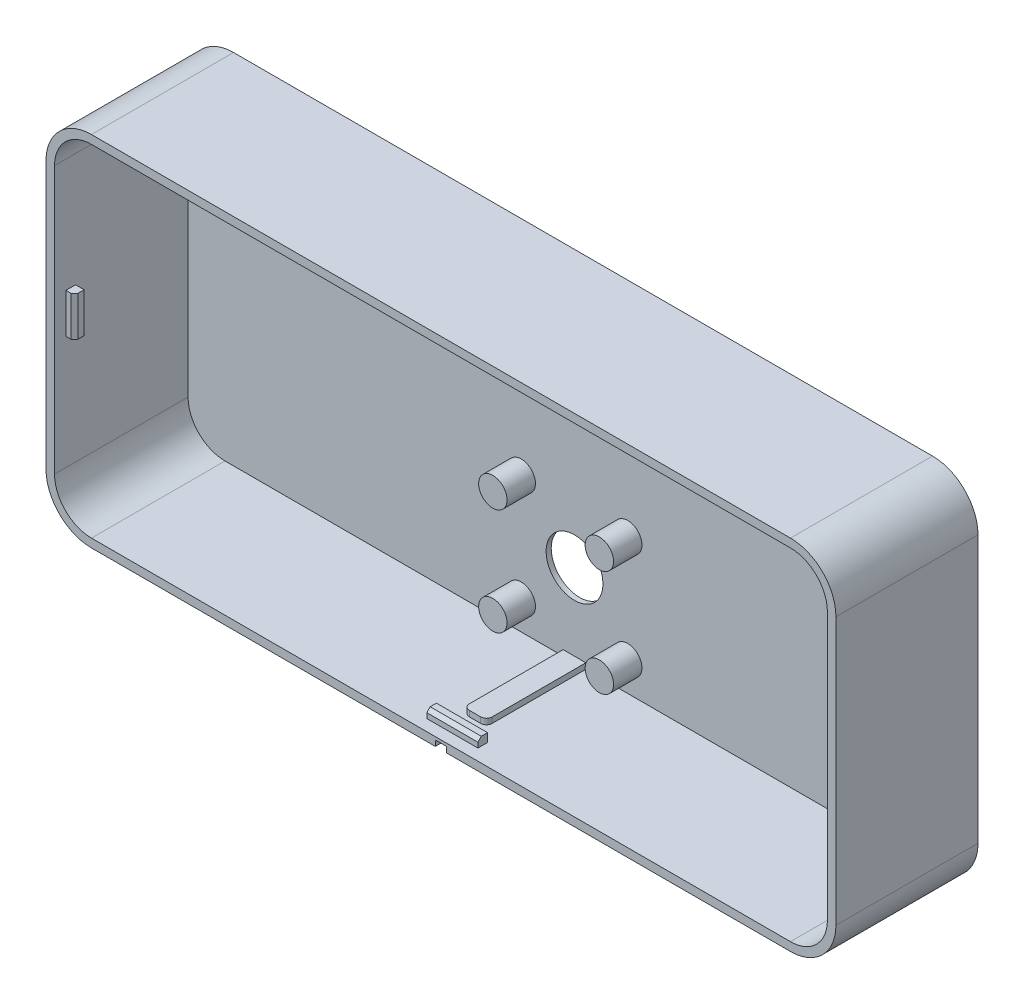
from build123d import *

# Parameters (mm, degrees)
BOSS_EXTRUDE1_DEPTH      = 25
SHELL1_T                 = -1.5
SKETCH2_W                = 9
SKETCH2_H                = 1.7
BOSS_EXTRUDE2_DEPTH      = 1.5
CHAMFER1_SIZE            = 0.6
CHAMFER1_OF_MIRROR1_SIZE = 0.6
SKETCH3_W                = 4
SKETCH3_H                = 17.5
BOSS_EXTRUDE3_DEPTH      = 1
SKETCH6_R                = 10.15
CUT_EXTRUDE3_DEPTH       = 0.6
SKETCH10_R               = 5
CUT_EXTRUDE4_DEPTH       = 81.111547233
SKETCH11_R               = 8
SKETCH11_R_2             = 7
BOSS_EXTRUDE5_DEPTH      = 0.6
SKETCH13_R               = 2.5
BOSS_EXTRUDE6_DEPTH      = 5
CUT_EXTRUDE5_START       = -2
SKETCH15_R               = 0.5
CUT_EXTRUDE5_DEPTH       = 77.515921952
SKETCH16_W               = 2
SKETCH16_H               = 58.164373892
CUT_EXTRUDE6_DEPTH       = 1
FILLET2_R                = 0.1
SKETCH17_R               = 15.5
SKETCH17_R_2             = 10.15
SKETCH17_R_3             = 0.5
BOSS_EXTRUDE7_DEPTH      = 1.2
SKETCH18_W               = 2
SKETCH18_H               = 1.626209188
CUT_EXTRUDE7_DEPTH       = 1
FILLET3_R                = 0.5
FILLET4_R                = 1
SKETCH19_W               = 1.7
SKETCH19_H               = 7
BOSS_EXTRUDE8_DEPTH      = 1.5
CHAMFER2_SIZE            = 0.6
CHAMFER2_OF_MIRROR2_SIZE = 0.6
FILLET5_R                = 0.2


with BuildPart() as part:
    # Sketch1 → Boss-Extrude1 (new body)
    with BuildSketch(Plane.XY):
        with BuildLine():
            Line((-61.5, 31.5), (61.5, 31.5))
            ThreePointArc((61.5, 31.5), (67.156854249, 29.156854249), (69.5, 23.5))
            Line((69.5, 23.5), (69.5, -23.5))
            ThreePointArc((69.5, -23.5), (67.156854249, -29.156854249), (61.5, -31.5))
            Line((61.5, -31.5), (-61.5, -31.5))
            ThreePointArc((-61.5, -31.5), (-67.156854249, -29.156854249), (-69.5, -23.5))
            Line((-69.5, -23.5), (-69.5, 23.5))
            ThreePointArc((-69.5, 23.5), (-67.156854249, 29.156854249), (-61.5, 31.5))
        make_face()
    extrude(amount=BOSS_EXTRUDE1_DEPTH)

    # Shell1
    shell1_openings = [part.faces().sort_by_distance(p)[0] for p in [
        (0, 0, 25),
    ]]
    offset(amount=SHELL1_T, openings=shell1_openings, kind=Kind.INTERSECTION)

    # Sketch2 → Boss-Extrude2 (add)
    with BuildSketch(Plane(origin=(0, 30, 0), x_dir=(-1, 0, 0), z_dir=(0, -1, 0))):
        with Locations((0, -22.15)):
            Rectangle(SKETCH2_W, SKETCH2_H)
    boss_extrude2 = extrude(amount=BOSS_EXTRUDE2_DEPTH)

    # Chamfer1
    chamfer1_edges = [part.edges().sort_by_distance(p)[0] for p in [
        (0, 28.5, 23),
    ]]
    chamfer(chamfer1_edges, length=CHAMFER1_SIZE)

    # Mirror1: Boss-Extrude2 across plane
    add(boss_extrude2.mirror(Plane.ZX))

    # Chamfer1 of Mirror1
    chamfer1_of_mirror1_edges = [part.edges().sort_by_distance(p)[0] for p in [
        (0, -28.5, 23),
    ]]
    chamfer(chamfer1_of_mirror1_edges, length=CHAMFER1_OF_MIRROR1_SIZE)

    # Sketch3 → Boss-Extrude3 (add)
    with BuildSketch(Plane(origin=(0, -30, 0), x_dir=(1, 0, 0), z_dir=(0, 1, 0))):
        with Locations((0, -10.25)):
            Rectangle(SKETCH3_W, SKETCH3_H)
    extrude(amount=BOSS_EXTRUDE3_DEPTH)

    # Sketch6 → Cut-Extrude3 (cut)
    with BuildSketch(Plane(origin=(0, 0, 0), x_dir=(-1, 0, 0), z_dir=(0, 0, -1))):
        with Locations((0, -15.5)):
            Circle(SKETCH6_R)
    extrude(amount=-CUT_EXTRUDE3_DEPTH, mode=Mode.SUBTRACT)

    # Sketch10 → Cut-Extrude4 (cut, through all)
    with BuildSketch(Plane(origin=(0, 0, 0.6), x_dir=(-1, 0, 0), z_dir=(0, 0, -1))):
        with Locations((0, -15.5)):
            Circle(SKETCH10_R)
    extrude(amount=-CUT_EXTRUDE4_DEPTH, mode=Mode.SUBTRACT)

    # Sketch11 → Boss-Extrude5 (add)
    with BuildSketch(Plane(origin=(0, 0, 0.6), x_dir=(-1, 0, 0), z_dir=(0, 0, -1))):
        with Locations((0, -15.5)):
            Circle(SKETCH11_R)
        with Locations((0, -15.5)):
            Circle(SKETCH11_R_2, mode=Mode.SUBTRACT)
    extrude(amount=BOSS_EXTRUDE5_DEPTH)

    # Sketch13 → Boss-Extrude6 (add)
    with BuildSketch(Plane.XY.offset(1.5)):
        with Locations((-9.369164851, -6.130835149)):
            Circle(SKETCH13_R)
        with Locations((9.369164851, -6.130835149)):
            Circle(SKETCH13_R)
        with Locations((9.369164851, -24.869164851)):
            Circle(SKETCH13_R)
        with Locations((-9.369164851, -24.869164851)):
            Circle(SKETCH13_R)
    extrude(amount=BOSS_EXTRUDE6_DEPTH)

    # Sketch15 → Cut-Extrude5 (cut, through all)
    with BuildSketch(Plane.XY.offset(6.5).offset(CUT_EXTRUDE5_START)):
        with Locations((9.369164851, -6.130835149)):
            Circle(SKETCH15_R)
        with Locations((-9.369164851, -6.130835149)):
            Circle(SKETCH15_R)
        with Locations((-9.369164851, -24.869164851)):
            Circle(SKETCH15_R)
        with Locations((9.369164851, -24.869164851)):
            Circle(SKETCH15_R)
    extrude(amount=-CUT_EXTRUDE5_DEPTH, mode=Mode.SUBTRACT)

    # Sketch16 → Cut-Extrude6 (cut)
    with BuildSketch(Plane(origin=(0, -31.5, 0), x_dir=(-1, 0, 0), z_dir=(0, -1, 0))):
        Rectangle(SKETCH16_W, SKETCH16_H)
    extrude(amount=-CUT_EXTRUDE6_DEPTH, mode=Mode.SUBTRACT)

    # Fillet2
    fillet2_edges = [part.edges().sort_by_distance(p)[0] for p in [
        (7, -15.5, 0.6),
        (8, -15.5, 0),
        (8, -15.5, 0.6),
        (7, -15.5, 0),
    ]]
    fillet(fillet2_edges, radius=FILLET2_R)

    # Sketch17 → Boss-Extrude7 (add)
    with BuildSketch(Plane(origin=(0, 0, 0), x_dir=(-1, 0, 0), z_dir=(0, 0, -1))):
        with Locations(Location((0, -15.5, 0), (0, 0, 266.300928937))):
            Circle(SKETCH17_R)
        with Locations((0, -15.5)):
            Circle(SKETCH17_R_2, mode=Mode.SUBTRACT)
        with Locations(Location((-9.369164851, -6.130835149, 0), (0, 0, 180))):
            Circle(SKETCH17_R_3, mode=Mode.SUBTRACT)
        with Locations(Location((9.369164851, -6.130835149, 0), (0, 0, 180))):
            Circle(SKETCH17_R_3, mode=Mode.SUBTRACT)
        with Locations(Location((9.369164851, -24.869164851, 0), (0, 0, 180))):
            Circle(SKETCH17_R_3, mode=Mode.SUBTRACT)
        with Locations(Location((-9.369164851, -24.869164851, 0), (0, 0, 180))):
            Circle(SKETCH17_R_3, mode=Mode.SUBTRACT)
    extrude(amount=BOSS_EXTRUDE7_DEPTH)

    # Sketch18 → Cut-Extrude7 (cut)
    with BuildSketch(Plane(origin=(0, -31.5, 0), x_dir=(-1, 0, 0), z_dir=(0, -1, 0))):
        with Locations((0, 0.813104594)):
            Rectangle(SKETCH18_W, SKETCH18_H)
    extrude(amount=-CUT_EXTRUDE7_DEPTH, mode=Mode.SUBTRACT)

    # Fillet3
    fillet3_edges = [part.edges().sort_by_distance(p)[0] for p in [
        (0, 0, 0),
    ]]
    fillet(fillet3_edges, radius=FILLET3_R)

    # Fillet4
    fillet4_edges = [part.edges().sort_by_distance(p)[0] for p in [
        (-2, -29.5, 19),
        (2, -29.5, 19),
    ]]
    fillet(fillet4_edges, radius=FILLET4_R)

    # Sketch19 → Boss-Extrude8 (add)
    with BuildSketch(Plane(origin=(-68, 0, 0), x_dir=(0, 0, -1), z_dir=(1, 0, 0))):
        with Locations((-22.15, 0)):
            Rectangle(SKETCH19_W, SKETCH19_H)
    boss_extrude8 = extrude(amount=BOSS_EXTRUDE8_DEPTH)

    # Chamfer2
    chamfer2_edges = [part.edges().sort_by_distance(p)[0] for p in [
        (-66.5, 0, 23),
    ]]
    chamfer(chamfer2_edges, length=CHAMFER2_SIZE)

    # Mirror2: Boss-Extrude8 across plane
    add(boss_extrude8.mirror(Plane(origin=(0, 0, 0), x_dir=(0, 0, 1), z_dir=(1, 0, 0))))

    # Chamfer2 of Mirror2
    chamfer2_of_mirror2_edges = [part.edges().sort_by_distance(p)[0] for p in [
        (66.5, 0, 23),
    ]]
    chamfer(chamfer2_of_mirror2_edges, length=CHAMFER2_OF_MIRROR2_SIZE)

    # Fillet5
    fillet5_edges = [part.edges().sort_by_distance(p)[0] for p in [
        (1, -30.5, 11.9),
        (-1, -30.5, 11.9),
    ]]
    fillet(fillet5_edges, radius=FILLET5_R)


solid = part.part
